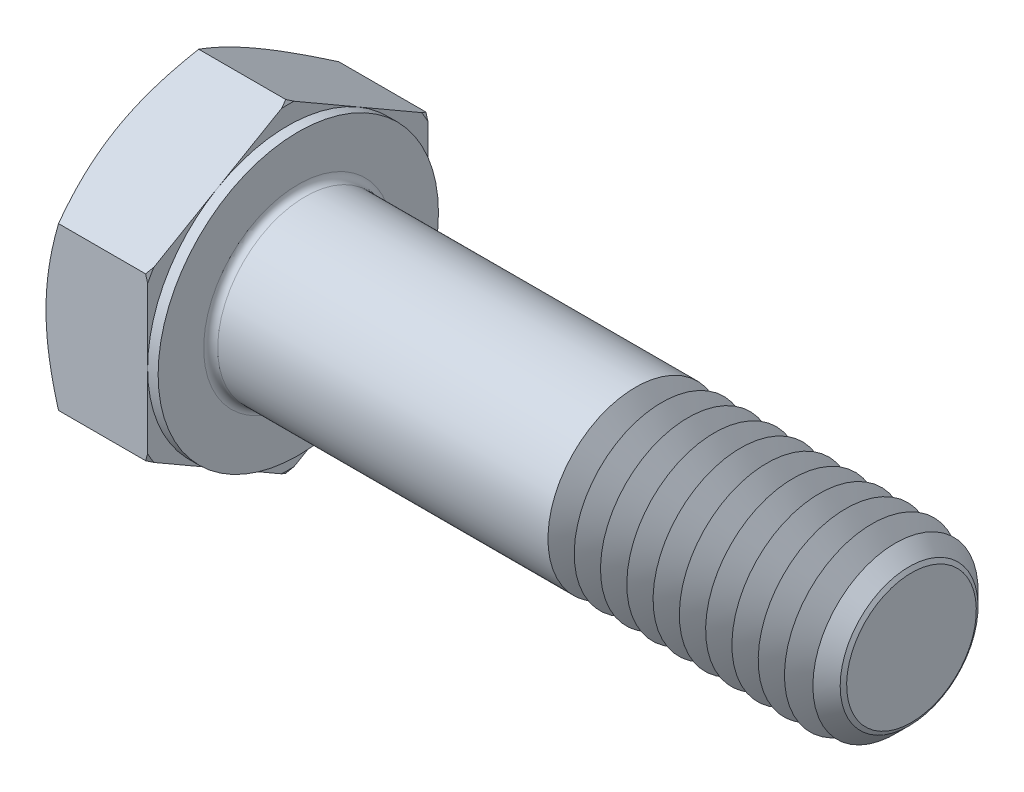
from build123d import *

# Parameters (mm, degrees)
EXTRUDE_378_DEPTH      = 6.4
SKETCH_4_W             = 0.6
SKETCH_4_H             = 11.237604307
CHAMFER_2060_SIZE      = 1.2
FILLET_2105_R          = 0.4
PATTERN_LINEAR_1_COUNT = 11
PATTERN_LINEAR_1_PITCH = 1.5


with BuildPart() as part:
    # 草图1 → Extrude 378 (new body)
    with BuildSketch(Plane(origin=(0, 0, 0), x_dir=(0, 0, -1), z_dir=(1, 0, 0))):
        Polygon((8, 4.618802154), (8, -4.618802154), (0, -9.237604307), (-8, -4.618802154), (-8, 4.618802154), (0, 9.237604307), align=None)
    extrude(amount=EXTRUDE_378_DEPTH)

    # 草图2 → 凸台-旋转1 (revolve)
    with BuildSketch(Plane.XY, mode=Mode.PRIVATE) as revolve_1_sk:
        Polygon((0, 0), (41.4, 0), (41.4, 3.701), (41.4, 5), (7.791693541, 5), (0, 5), align=None)
    revolve(revolve_1_sk.sketch.rotate(Axis((0, 0, 0), (1, 0, 0)), 90), axis=Axis((0, 0, 0), (1, 0, 0)))

    # 草图3 → 切除-旋转1 (revolve, cut)
    with BuildSketch(Plane.XY):
        Polygon((0, 8), (3.601282526, 14.237604307), (3.601282526, 19.237604307), (-10, 19.237604307), (-10, 8), align=None)
    revolve(axis=Axis((0, 0, 0), (1, 0, 0)), mode=Mode.SUBTRACT)

    # 草图5 → 切除-旋转2 (revolve, cut)
    with BuildSketch(Plane.XY):
        Polygon((6.4, 8), (2.798717474, 14.237604307), (2.798717474, 19.237604307), (12.798717474, 19.237604307), (12.798717474, 8), align=None)
    revolve(axis=Axis((0, 0, 0), (1, 0, 0)), mode=Mode.SUBTRACT)

    # 草图4 → 切除-旋转3 (revolve, cut)
    with BuildSketch(Plane.XY, mode=Mode.PRIVATE) as cut_revolve_3_sk:
        with Locations((6.1, 13.618802154)):
            Rectangle(SKETCH_4_W, SKETCH_4_H)
    revolve(cut_revolve_3_sk.sketch.rotate(Axis((0, 0, 0), (1, 0, 0)), 270), axis=Axis((0, 0, 0), (1, 0, 0)), mode=Mode.SUBTRACT)

    # Chamfer 2060
    chamfer_2060_edges = [part.edges().sort_by_distance(p)[0] for p in [
        (41.4, 0, -5),
    ]]
    chamfer(chamfer_2060_edges, length=CHAMFER_2060_SIZE)

    # Fillet 2105
    fillet_2105_edges = [part.edges().sort_by_distance(p)[0] for p in [
        (6.4, 0, -5),
    ]]
    fillet(fillet_2105_edges, radius=FILLET_2105_R)

    # 草图6 → 切除-旋转4 (revolve, cut)
    with BuildSketch(Plane.XY):
        Polygon((26.4, -3.701), (25.650022, -5), (25.650022, -6.25), (27.149978, -6.25), (27.149978, -5), align=None)
    cut_revolve_4 = revolve(axis=Axis((-3.175, 0, 0), (1, 0, 0)), mode=Mode.SUBTRACT)

    # 阵列(线性)1: 切除-旋转4 ×11
    with Locations(*[(i * PATTERN_LINEAR_1_PITCH, 0, 0) for i in range(1, PATTERN_LINEAR_1_COUNT)]):
        add(cut_revolve_4, mode=Mode.SUBTRACT)


solid = part.part
